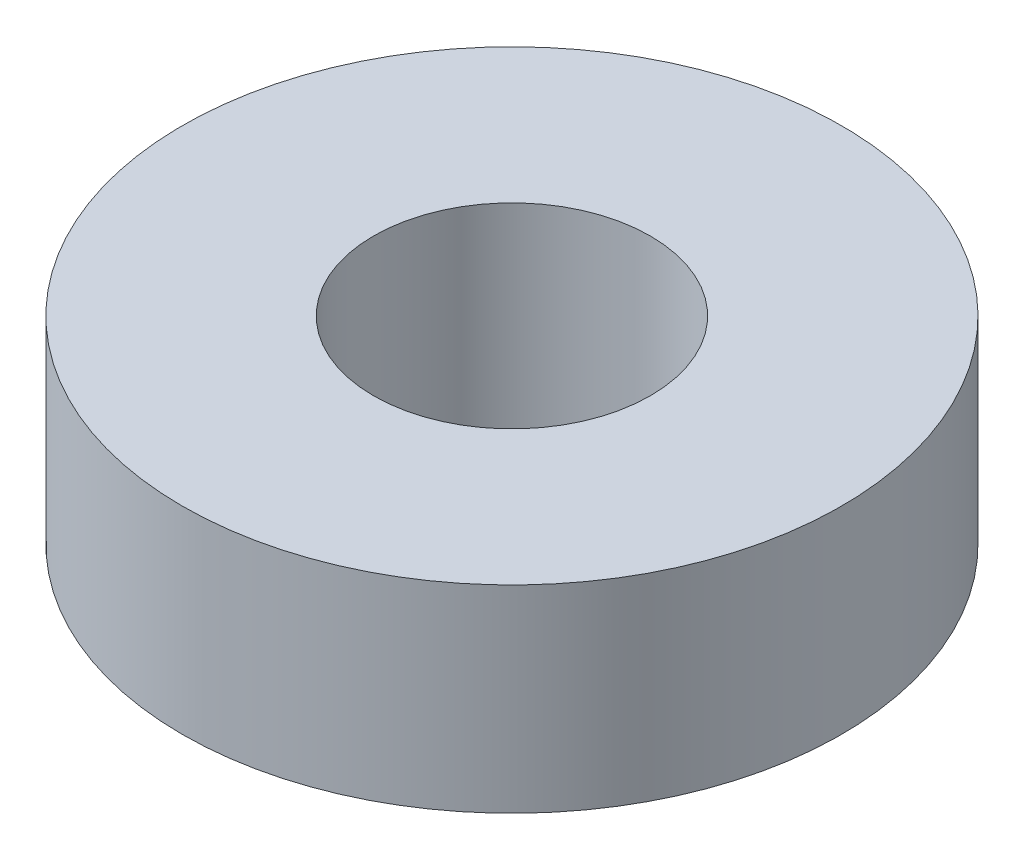
from build123d import *

# Parameters (mm, degrees)
SKETCH_1_R      = 5
SKETCH_1_R_2    = 2.1
EXTRUDE_1_DEPTH = 3


with BuildPart() as part:
    # 草图1 → 凸台-拉伸1 (new body)
    with BuildSketch(Plane(origin=(0, 0, 0), x_dir=(1, 0, 0), z_dir=(0, 1, 0))):
        with Locations(Location((0, 0, 0), (0, 0, 270))):
            Circle(SKETCH_1_R)
        with Locations(Location((0, 0, 0), (0, 0, 270))):
            Circle(SKETCH_1_R_2, mode=Mode.SUBTRACT)
    extrude(amount=EXTRUDE_1_DEPTH)


solid = part.part
